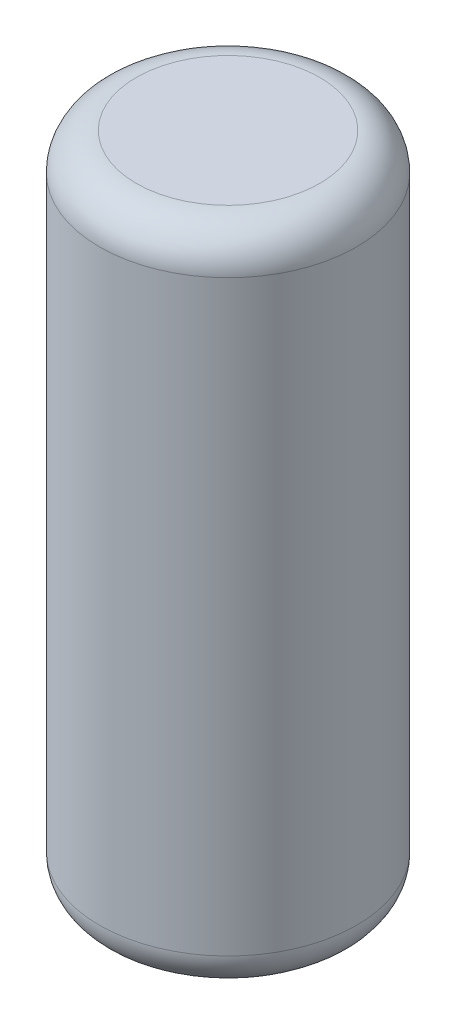
SolidWorks part; units mm, degrees
material "AISI 1045 钢，冷拔"
ref_plane "Front Plane" through (0, 0, 0) normal (0, 0, 1) x (1, 0, 0)
ref_plane "Top Plane" through (0, 0, 0) normal (0, 1, 0) x (1, 0, 0)
ref_plane "Right Plane" through (0, 0, 0) normal (1, 0, 0) x (0, 0, -1)
sketch "Sketch1" plane through (0, 0, 0) normal (0, 1, 0) x (1, 0, 0)
  circle A0 centre (0, 0) radius 3.5
extrude "Boss-Extrude1" add sketch "Sketch1" along normal blind 18
fillet "Fillet1" radius 1 2 edges at (0, 0, 3.5) (0, 18, 3.5)
